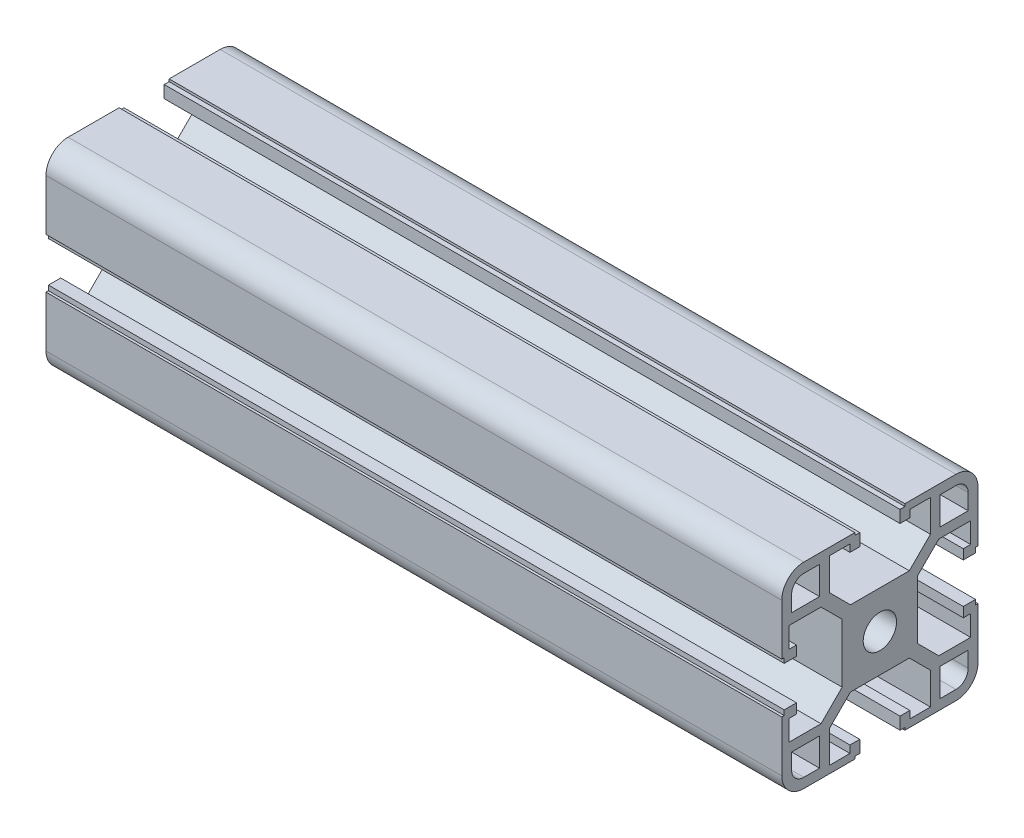
from build123d import *

# Parameters (mm, degrees)
SKETCH1_R                                = 3.4
ALUMINUM_PROFILE_40_X_40B_X_R4_5_1_DEPTH = 150


with BuildPart() as part:
    # Sketch1 → Aluminum profile 40 X 40B X R4.5(1) (new body)
    with BuildSketch(Plane.YZ):
        with BuildLine():
            Line((-5.1, 20), (-5.1, 19.5))
            Line((-5.1, 19.5), (-4.1, 19.5))
            Line((-4.1, 19.5), (-4.1, 17))
            Line((-4.1, 17), (-6.1, 17))
            Line((-6.1, 17), (-6.1, 18.5))
            Line((-6.1, 18.5), (-10.3, 18.5))
            Line((-10.3, 18.5), (-10.3, 12))
            Line((-10.3, 12), (-6, 7.7))
            Line((-6, 7.7), (6, 7.7))
            Line((6, 7.7), (10.3, 12))
            Line((10.3, 12), (10.3, 18.5))
            Line((10.3, 18.5), (6.1, 18.5))
            Line((6.1, 18.5), (6.1, 17))
            Line((6.1, 17), (4.1, 17))
            Line((4.1, 17), (4.1, 19.5))
            Line((4.1, 19.5), (5.1, 19.5))
            Line((5.1, 19.5), (5.1, 20))
            Line((5.1, 20), (15.5, 20))
            ThreePointArc((15.5, 20), (18.681980515, 18.681980515), (20, 15.5))
            Line((20, 15.5), (20, 5.1))
            Line((20, 5.1), (19.5, 5.1))
            Line((19.5, 5.1), (19.5, 4.1))
            Line((19.5, 4.1), (17, 4.1))
            Line((17, 4.1), (17, 6.1))
            Line((17, 6.1), (18.5, 6.1))
            Line((18.5, 6.1), (18.5, 10.3))
            Line((18.5, 10.3), (12, 10.3))
            Line((12, 10.3), (7.7, 6))
            Line((7.7, 6), (7.7, -6))
            Line((7.7, -6), (12, -10.3))
            Line((12, -10.3), (18.5, -10.3))
            Line((18.5, -10.3), (18.5, -6.1))
            Line((18.5, -6.1), (17, -6.1))
            Line((17, -6.1), (17, -4.1))
            Line((17, -4.1), (19.5, -4.1))
            Line((19.5, -4.1), (19.5, -5.1))
            Line((19.5, -5.1), (20, -5.1))
            Line((20, -5.1), (20, -15.5))
            ThreePointArc((20, -15.5), (18.681980515, -18.681980515), (15.5, -20))
            Line((15.5, -20), (5.1, -20))
            Line((5.1, -20), (5.1, -19.5))
            Line((5.1, -19.5), (4.1, -19.5))
            Line((4.1, -19.5), (4.1, -17))
            Line((4.1, -17), (6.1, -17))
            Line((6.1, -17), (6.1, -18.5))
            Line((6.1, -18.5), (10.3, -18.5))
            Line((10.3, -18.5), (10.3, -12))
            Line((10.3, -12), (6, -7.7))
            Line((6, -7.7), (-6, -7.7))
            Line((-6, -7.7), (-10.3, -12))
            Line((-10.3, -12), (-10.3, -18.5))
            Line((-10.3, -18.5), (-6.1, -18.5))
            Line((-6.1, -18.5), (-6.1, -17))
            Line((-6.1, -17), (-4.1, -17))
            Line((-4.1, -17), (-4.1, -19.5))
            Line((-4.1, -19.5), (-5.1, -19.5))
            Line((-5.1, -19.5), (-5.1, -20))
            Line((-5.1, -20), (-15.5, -20))
            ThreePointArc((-15.5, -20), (-18.681980515, -18.681980515), (-20, -15.5))
            Line((-20, -15.5), (-20, -5.1))
            Line((-20, -5.1), (-19.5, -5.1))
            Line((-19.5, -5.1), (-19.5, -4.1))
            Line((-19.5, -4.1), (-17, -4.1))
            Line((-17, -4.1), (-17, -6.1))
            Line((-17, -6.1), (-18.5, -6.1))
            Line((-18.5, -6.1), (-18.5, -10.3))
            Line((-18.5, -10.3), (-12, -10.3))
            Line((-12, -10.3), (-7.7, -6))
            Line((-7.7, -6), (-7.7, 6))
            Line((-7.7, 6), (-12, 10.3))
            Line((-12, 10.3), (-18.5, 10.3))
            Line((-18.5, 10.3), (-18.5, 6.1))
            Line((-18.5, 6.1), (-17, 6.1))
            Line((-17, 6.1), (-17, 4.1))
            Line((-17, 4.1), (-19.5, 4.1))
            Line((-19.5, 4.1), (-19.5, 5.1))
            Line((-19.5, 5.1), (-20, 5.1))
            Line((-20, 5.1), (-20, 15.5))
            ThreePointArc((-20, 15.5), (-18.681980515, 18.681980515), (-15.5, 20))
            Line((-15.5, 20), (-5.1, 20))
        make_face()
        Circle(SKETCH1_R, mode=Mode.SUBTRACT)
        with BuildLine():
            Line((12.3, 18), (15.5, 18))
            ThreePointArc((15.5, 18), (17.267766953, 17.267766953), (18, 15.5))
            Line((18, 15.5), (18, 12.3))
            Line((18, 12.3), (12.3, 12.3))
            Line((12.3, 12.3), (12.3, 18))
        make_face(mode=Mode.SUBTRACT)
        with BuildLine():
            Line((-15.5, 18), (-12.3, 18))
            Line((-12.3, 18), (-12.3, 12.3))
            Line((-12.3, 12.3), (-18, 12.3))
            Line((-18, 12.3), (-18, 15.5))
            ThreePointArc((-18, 15.5), (-17.267766953, 17.267766953), (-15.5, 18))
        make_face(mode=Mode.SUBTRACT)
        with BuildLine():
            Line((-18, -12.3), (-12.3, -12.3))
            Line((-12.3, -12.3), (-12.3, -18))
            Line((-12.3, -18), (-15.5, -18))
            ThreePointArc((-15.5, -18), (-17.267766953, -17.267766953), (-18, -15.5))
            Line((-18, -15.5), (-18, -12.3))
        make_face(mode=Mode.SUBTRACT)
        with BuildLine():
            Line((12.3, -12.3), (18, -12.3))
            Line((18, -12.3), (18, -15.5))
            ThreePointArc((18, -15.5), (17.267766953, -17.267766953), (15.5, -18))
            Line((15.5, -18), (12.3, -18))
            Line((12.3, -18), (12.3, -12.3))
        make_face(mode=Mode.SUBTRACT)
    extrude(amount=ALUMINUM_PROFILE_40_X_40B_X_R4_5_1_DEPTH)


solid = part.part
